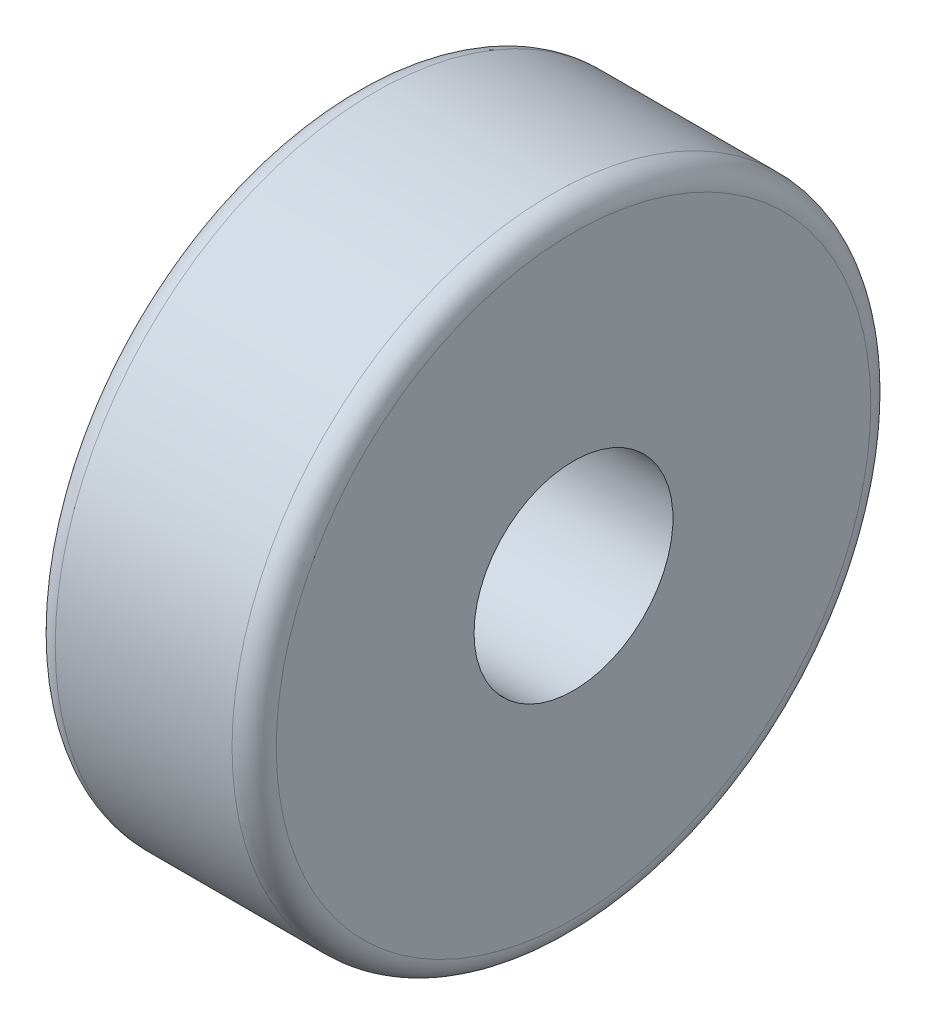
SolidWorks part; units mm, degrees
ref_plane "Front Plane" through (0, 0, 0) normal (0, 0, 1) x (1, 0, 0)
ref_plane "Top Plane" through (0, 0, 0) normal (0, 1, 0) x (1, 0, 0)
ref_plane "Right Plane" through (0, 0, 0) normal (1, 0, 0) x (0, 0, -1)
sketch "Sketch 1" plane through (0, 0, 0) normal (0, 0, 1) x (1, 0, 0)
  line L0 (0, 159.8315) -> (0, -117.6966) construction
  line L1 (-106.1798, 0) -> (75.2809, 0) construction
  line L3 (-50, 45) -> (50, 45)
  line L4 (-50, 45) -> (-50, 144.5)
  line L5 (-50, 144.5) -> (50, 144.5)
  line L6 (50, 45) -> (50, 144.5)
  line L7 (-50, 45) -> (50, 144.5) construction
  line L8 (-50, 144.5) -> (50, 45) construction
  point P5 (0, 94.75)
  dimension "D1" = 90
  dimension "D2" = 144.5
  dimension "D3" = 100
revolve "Revolve 1" add sketch "Sketch 1" angle 360 about L1
fillet "Fillet 1" radius 10 2 edges at (50, 0, 144.5) (-50, 0, 144.5)
